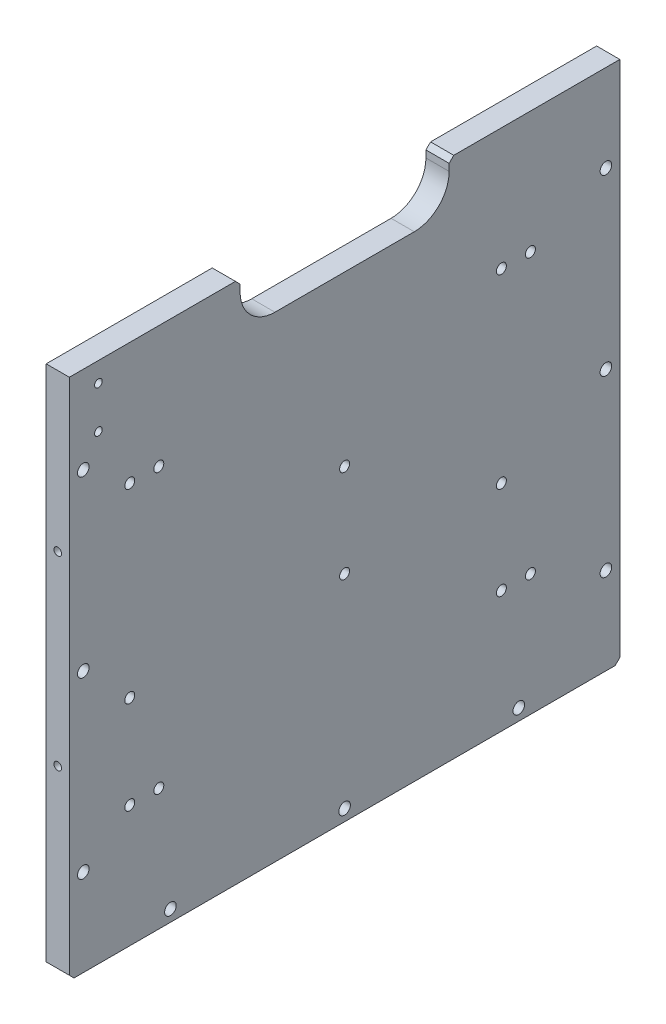
SolidWorks part; units mm, degrees
material "电木（PF）"
ref_plane "前视基准面" through (0, 0, 0) normal (0, 0, 1) x (1, 0, 0)
ref_plane "上视基准面" through (0, 0, 0) normal (0, 1, 0) x (1, 0, 0)
ref_plane "右视基准面" through (0, 0, 0) normal (1, 0, 0) x (0, 0, -1)
sketch "草图1" plane through (0, 0, 0) normal (1, 0, 0) x (0, 0, -1)
  line L1 (-118.5, 125) -> (118.5, 125)
  line L2 (-118.5, 125) -> (-118.5, -125)
  line L3 (-118.5, -125) -> (118.5, -125)
  line L4 (118.5, 125) -> (118.5, -125)
  line L5 (-118.5, 125) -> (118.5, -125) construction
  line L6 (-118.5, -125) -> (118.5, 125) construction
  point P0 (0, 0)
  dimension "D1" = 237
  dimension "D2" = 250
extrude "凸台-拉伸1" add sketch "草图1" along normal mid plane 10
other "移动面1" face at (0, 125, 0) parameters "D1"=17.5
other "移动面2" face at (0, -125, 0) parameters "D1"=7.5
hole_wizard "M4 螺纹孔1" positions "草图2" profile "草图3" tap size "M4" standard "GB"
sketch "草图2" plane through (0, 0, 118.5) normal (0, 0, 1) x (1, 0, 0)
  point P0 (0, -40)
  point P3 (0, 40)
cosmetic thread "孔螺蚊线1" parameters "D1"=8, "D2"=4
cosmetic thread "孔螺蚊线2" parameters "D1"=8, "D2"=4
sketch "草图3" plane through (0, -40, 118.5) normal (1, 0, 0) x (0, -1, 0)
  line L0 (0, 0) -> (0, 11.0914)
  line L1 (0, 11.0914) -> (1.65, 10.1)
  line L2 (1.65, 10.1) -> (1.65, 0)
  line L5 (1.65, 0) -> (0, 0)
  line L10 (0, 11.0914) -> (-1.65, 10.1) construction
  line L11 (0, -6.35) -> (0, 107.95) construction
  dimension "螺纹孔钻头直径" = 3.3
  dimension "螺纹孔钻头深度" = 10.1
  dimension "导头角度" = 118
mirror "镜向1" about plane through (0, 0, 0) normal (0, 0, 1) of "M4 螺纹孔1"
hole_wizard "M4 螺纹孔2" positions "草图4" profile "草图5" tap size "M4" standard "GB" end condition through all
sketch "草图4" plane through (5, 0, 0) normal (1, 0, 0) x (0, 0, -1)
  point P0 (-106, 99)
  point P3 (-106, 81)
sketch "草图5" plane through (5, 99, 106) normal (0, 1, 0) x (0, 0, -1)
  line L0 (0, 0) -> (0, 10)
  line L1 (0, 10) -> (1.65, 10)
  line L2 (1.65, 10) -> (1.65, 0)
  line L5 (1.65, 0) -> (0, 0)
  line L11 (0, -6.35) -> (0, 107.95) construction
  dimension "通孔螺纹孔钻头直径" = 3.3
  dimension "通孔螺纹孔钻头深度" = 10
cosmetic thread "孔螺蚊线3" parameters "D2"=4
cosmetic thread "孔螺蚊线4" parameters "D2"=4
hole_wizard "M6 螺纹孔1" positions "草图6" profile "草图8" tap size "M6" standard "GB" end condition through all
sketch "草图6" plane through (-5, 0, 0) normal (-1, 0, 0) x (0, 0, 1)
  point P0 (-112.5, 70)
  point P3 (-112.5, -5)
  point P6 (-112.5, -80)
sketch "草图8" plane through (-5, 70, -112.5) normal (0, 1, 0) x (0, 0, 1)
  line L0 (0, 0) -> (0, 10)
  line L1 (0, 10) -> (2.5, 10)
  line L2 (2.5, 10) -> (2.5, 0)
  line L5 (2.5, 0) -> (0, 0)
  line L11 (0, -6.35) -> (0, 107.95) construction
  dimension "通孔螺纹孔钻头直径" = 5
  dimension "通孔螺纹孔钻头深度" = 10
cosmetic thread "孔螺蚊线5" parameters "D2"=6
cosmetic thread "孔螺蚊线6" parameters "D2"=6
cosmetic thread "孔螺蚊线7" parameters "D2"=6
mirror "镜向2" about plane through (0, 0, 0) normal (0, 0, 1) of "M6 螺纹孔1"
hole_wizard "M6 螺纹孔2" positions "草图9" profile "草图10" tap size "M6" standard "GB" end condition through all
sketch "草图9" plane through (-5, 0, 0) normal (-1, 0, 0) x (0, 0, 1)
  point P0 (75, -112.5)
  point P3 (0, -112.5)
  point P6 (-75, -112.5)
sketch "草图10" plane through (-5, -112.5, 75) normal (0, 1, 0) x (0, 0, 1)
  line L0 (0, 0) -> (0, 10)
  line L1 (0, 10) -> (2.5, 10)
  line L2 (2.5, 10) -> (2.5, 0)
  line L5 (2.5, 0) -> (0, 0)
  line L11 (0, -6.35) -> (0, 107.95) construction
  dimension "通孔螺纹孔钻头直径" = 5
  dimension "通孔螺纹孔钻头深度" = 10
cosmetic thread "孔螺蚊线8" parameters "D2"=6
cosmetic thread "孔螺蚊线9" parameters "D2"=6
cosmetic thread "孔螺蚊线10" parameters "D2"=6
chamfer "倒角1" distance 2 angle 45 2 edges at (0, -117.5, -118.5) (0, -117.5, 118.5)
sketch "草图11" plane through (-5, 0, 0) normal (-1, 0, 0) x (0, 0, 1)
  line L0 (0, 0) -> (0, 184.7888) construction
  line L1 (-118.5, 107.5) -> (118.5, 107.5) construction
  line L2 (-45, 148.58) -> (45, 148.58)
  line L3 (-45, 148.58) -> (-45, 102.5)
  line L4 (-30, 87.5) -> (30, 87.5)
  line L5 (45, 148.58) -> (45, 102.5)
  line L6 (-45, 148.58) -> (45, 87.5) construction
  line L7 (-45, 87.5) -> (45, 148.58) construction
  arc A0 (45, 102.5) -> (30, 87.5) centre (30, 102.5) cw
  arc A1 (-30, 87.5) -> (-45, 102.5) centre (-30, 102.5) cw
  point P3 (0, 118.04)
  dimension "D3" = 15
  dimension "D1" = 20
  dimension "D2" = 90
extrude "切除-拉伸1" cut sketch "草图11" against normal blind 71
chamfer "倒角2" distance 2 angle 45 2 edges at (0, 107.5, -45) (0, 107.5, 45)
hole_wizard "打孔尺寸(%根据)开槽圆柱头螺钉的类型1" positions "草图12" profile "草图14" counterbore size "M4" standard "GB" end condition through all
sketch "草图12" plane through (-5, 0, 0) normal (-1, 0, 0) x (0, 0, 1)
  point P0 (-67.5, 55)
  point P2 (92.5, 55)
  point P4 (92.5, -65)
  point P6 (-67.5, -65)
  point P8 (-67.5, -25)
  point P10 (92.5, -25)
sketch "草图14" plane through (-5, 55, -67.5) normal (0, 1, 0) x (0, 0, 1)
  line L0 (0, 0) -> (0, 10)
  line L1 (0, 10) -> (2.15, 10)
  line L3 (2.15, 10) -> (2.15, 4.6)
  line L4 (2.15, 4.6) -> (4, 4.6)
  line L5 (4, 4.6) -> (4, 0)
  line L7 (4, 0) -> (0, 0)
  line L11 (0, -6.35) -> (0, 107.95) construction
  dimension "通孔孔直径" = 4.3
  dimension "通孔孔深度" = 10
  dimension "柱形沉头孔直径" = 8
  dimension "柱形沉头孔深度" = 4.6
hole_wizard "打孔尺寸(%根据)内六角圆柱头螺钉的类型1" positions "草图17" profile "草图20" counterbore size "M4" standard "GB" end condition through all
sketch "草图17" plane through (-5, 0, 0) normal (-1, 0, 0) x (0, 0, 1)
  point P0 (80, 55)
  point P2 (-80, 55)
  point P4 (-80, -65)
  point P6 (80, -65)
  point P8 (0, -25)
  point P10 (0, 15)
sketch "草图20" plane through (-5, 55, 80) normal (0, 1, 0) x (0, 0, 1)
  line L0 (0, 0) -> (0, 10)
  line L1 (0, 10) -> (2.15, 10)
  line L3 (2.15, 10) -> (2.15, 5)
  line L4 (2.15, 5) -> (4, 5)
  line L5 (4, 5) -> (4, 0)
  line L7 (4, 0) -> (0, 0)
  line L11 (0, -6.35) -> (0, 107.95) construction
  dimension "通孔孔直径" = 4.3
  dimension "通孔孔深度" = 10
  dimension "柱形沉头孔直径" = 8
  dimension "柱形沉头孔深度" = 5
